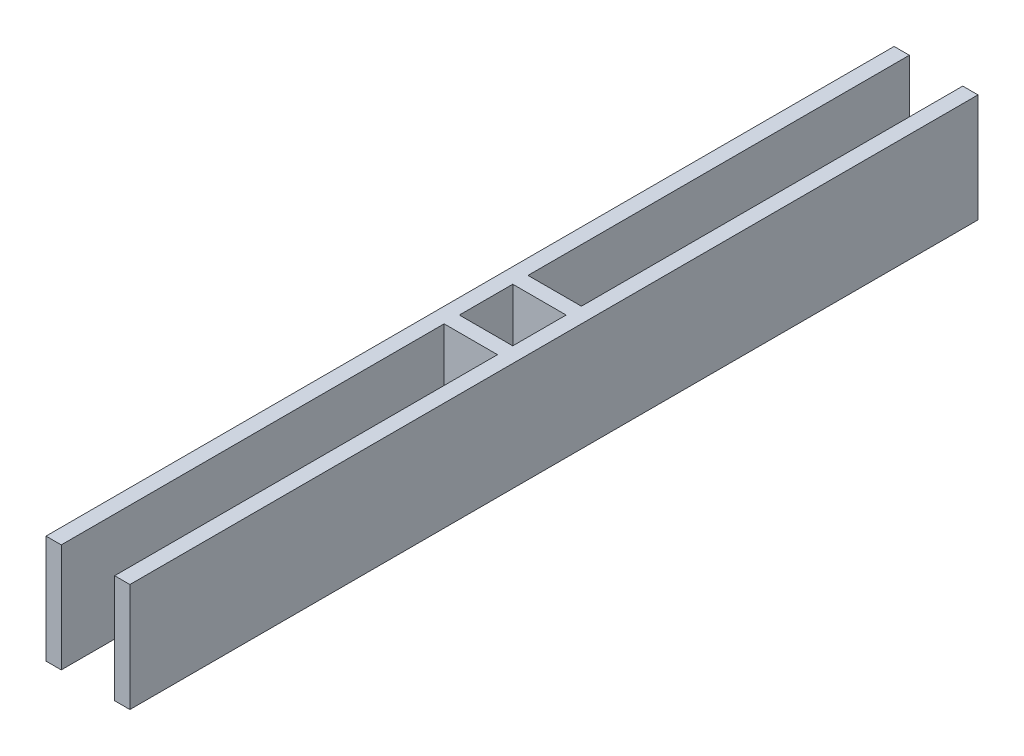
from build123d import *

# Parameters (mm, degrees)
SKETCH1_W           = 10
SKETCH1_H           = 71
BOSS_EXTRUDE1_DEPTH = 556
SKETCH2_W           = 10
SKETCH2_H           = 71
BOSS_EXTRUDE2_DEPTH = 35
SKETCH3_W           = 10
SKETCH3_H           = 556
BOSS_EXTRUDE3_DEPTH = 71


with BuildPart() as part:
    # Sketch1 → Boss-Extrude1 (new body)
    with BuildSketch(Plane.XY):
        Rectangle(SKETCH1_W, SKETCH1_H)
    extrude(amount=BOSS_EXTRUDE1_DEPTH)

    # Sketch2 → Boss-Extrude2 (add)
    with BuildSketch(Plane(origin=(5, 0, 0), x_dir=(0, 0, -1), z_dir=(1, 0, 0))):
        with Locations((-300, 0)):
            Rectangle(SKETCH2_W, SKETCH2_H)
        with Locations((-255, 0)):
            Rectangle(SKETCH2_W, SKETCH2_H)
    extrude(amount=BOSS_EXTRUDE2_DEPTH)

    # Sketch3 → Boss-Extrude3 (add)
    with BuildSketch(Plane(origin=(0, 35.5, 0), x_dir=(1, 0, 0), z_dir=(0, 1, 0))):
        with Locations((45, -278)):
            Rectangle(SKETCH3_W, SKETCH3_H)
    extrude(amount=-BOSS_EXTRUDE3_DEPTH)


solid = part.part
